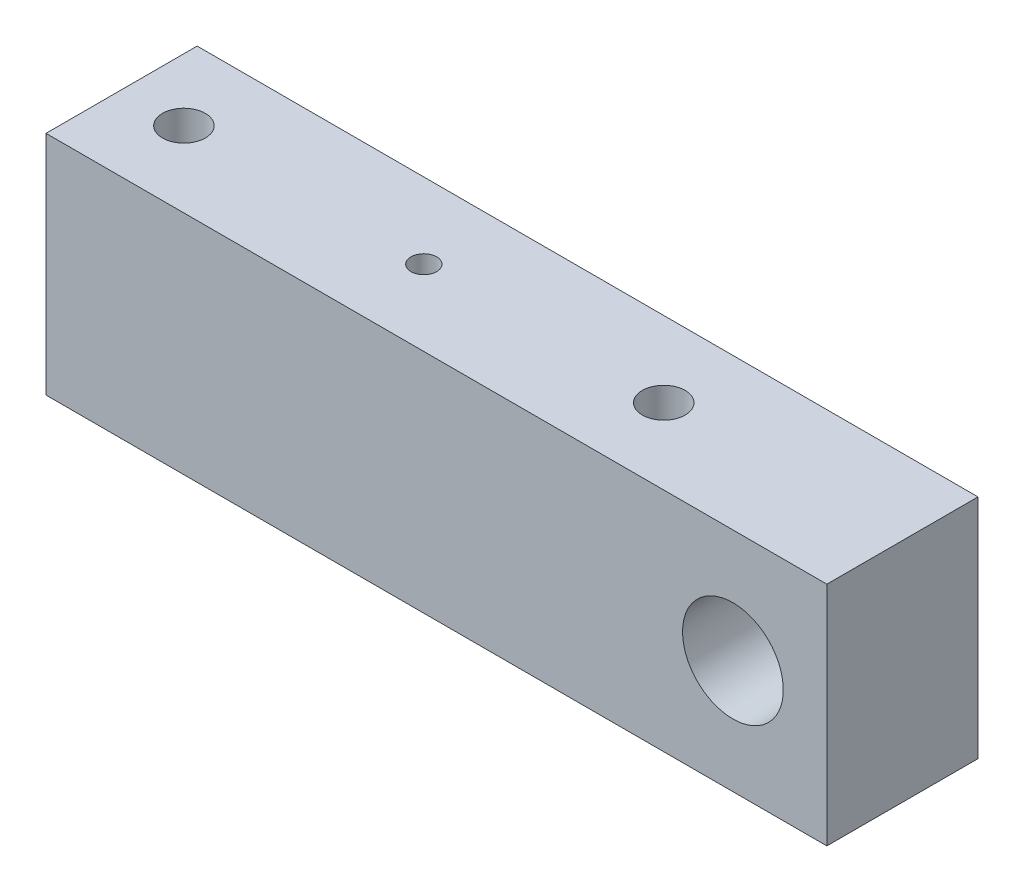
from build123d import *

# Parameters (mm, degrees)
SKETCH_1_W              = 310
SKETCH_1_H              = 90
EXTRUDE_1_DEPTH         = 60
SKETCH_2_R              = 8.5
CUT_EXTRUDE_1_DEPTH     = 90
HOLE_WIZARD_M12_1_D     = 10.2
HOLE_WIZARD_M12_1_DEPTH = 30.25
HOLE_WIZARD_M12_1_TIP   = 3.064389157
SKETCH_6_R              = 20
CUT_EXTRUDE_2_DEPTH     = 60


with BuildPart() as part:
    # 草图1 → 凸台-拉伸1 (new body)
    with BuildSketch(Plane.XY):
        Rectangle(SKETCH_1_W, SKETCH_1_H)
    extrude(amount=EXTRUDE_1_DEPTH)

    # 草图2 → 切除-拉伸1 (cut)
    with BuildSketch(Plane(origin=(0, 45, 0), x_dir=(1, 0, 0), z_dir=(0, 1, 0))):
        with Locations(Location((-130.25, -30, 0), (0, 0, 180))):
            Circle(SKETCH_2_R)
        with Locations(Location((60.25, -30, 0), (0, 0, 180))):
            Circle(SKETCH_2_R)
    extrude(amount=-CUT_EXTRUDE_1_DEPTH, mode=Mode.SUBTRACT)

    # M12 螺纹孔1
    with Locations(Plane(origin=(0, 45, 0), x_dir=(1, 0, 0), z_dir=(0, 1, 0))):
        with Locations((-35, -30)):
            Hole(HOLE_WIZARD_M12_1_D / 2, depth=HOLE_WIZARD_M12_1_DEPTH)
            with Locations((0, 0, -(HOLE_WIZARD_M12_1_DEPTH + HOLE_WIZARD_M12_1_TIP / 2))):  # 118° drill point
                Cone(0, HOLE_WIZARD_M12_1_D / 2, HOLE_WIZARD_M12_1_TIP, mode=Mode.SUBTRACT)

    # 草图6 → 切除-拉伸2 (cut)
    with BuildSketch(Plane(origin=(0, 0, 0), x_dir=(-1, 0, 0), z_dir=(0, 0, -1))):
        with Locations((-117.7, 0)):
            Circle(SKETCH_6_R)
    extrude(amount=-CUT_EXTRUDE_2_DEPTH, mode=Mode.SUBTRACT)


solid = part.part
